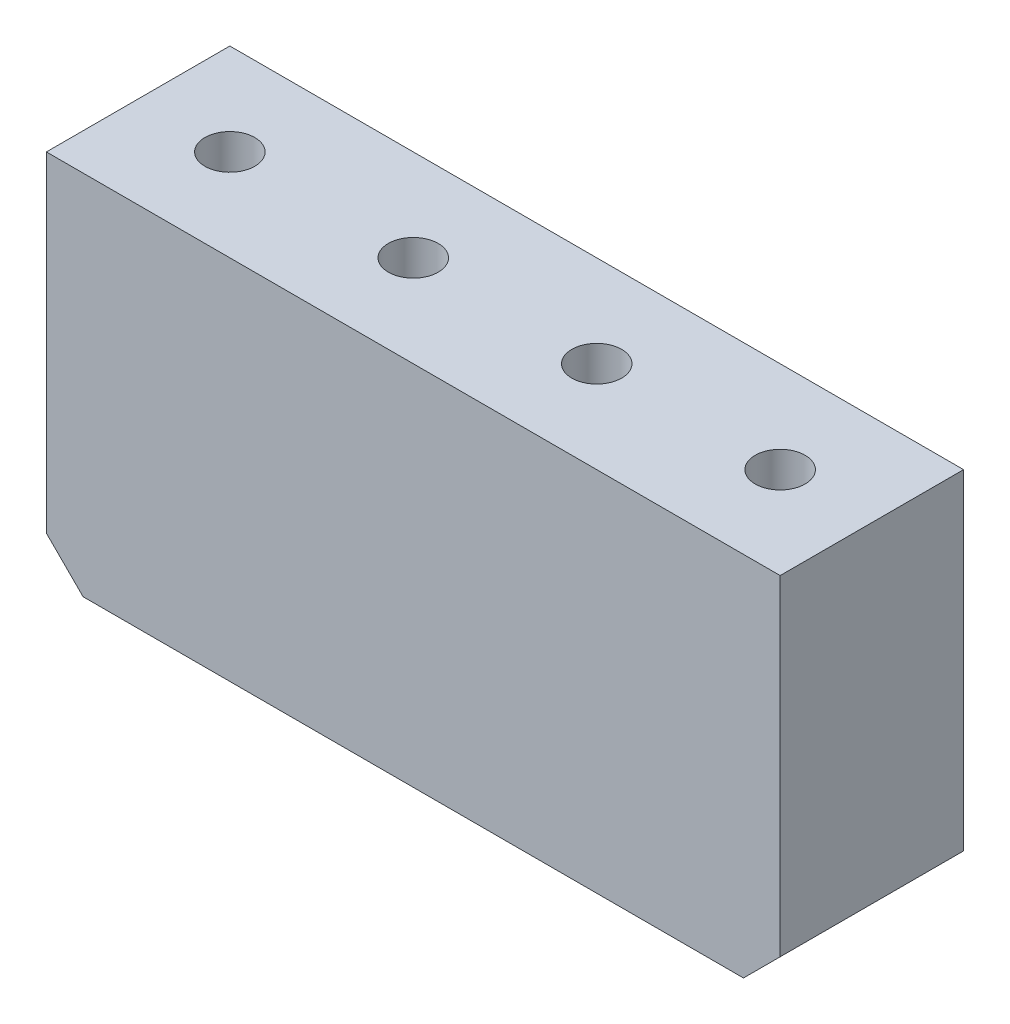
SolidWorks part; units mm, degrees
material "1023 碳钢板 (SS)"
ref_plane "Front Plane" through (0, 0, 0) normal (0, 0, 1) x (1, 0, 0)
ref_plane "Top Plane" through (0, 0, 0) normal (0, 1, 0) x (1, 0, 0)
ref_plane "Right Plane" through (0, 0, 0) normal (1, 0, 0) x (0, 0, -1)
sketch "Sketch1" plane through (0, 0, 0) normal (0, 0, 1) x (1, 0, 0)
  line L1 (-50, 25) -> (50, 25)
  line L2 (-50, 25) -> (-50, -25)
  line L3 (-50, -25) -> (50, -25)
  line L4 (50, 25) -> (50, -25)
  line L5 (-50, 25) -> (50, -25) construction
  line L6 (-50, -25) -> (50, 25) construction
  point P0 (0, 0)
  dimension "D1" = 100
  dimension "D2" = 50
extrude "Boss-Extrude1" add sketch "Sketch1" along normal blind 25 contours L2 L1 L4 L3
sketch "Sketch2" plane through (0, 25, 0) normal (0, 1, 0) x (1, 0, 0)
  line L0 (-50, -25) -> (-50, 0) construction
  circle A0 centre (-37.5, -12.5) radius 2.8145
  circle A1 centre (-12.5, -12.5) radius 3.8665
  circle A2 centre (37.5, -12.5) radius 5.7881
  circle A3 centre (12.5, -12.5) radius 3.4368
  point P12 (-50, -12.5)
  dimension "D1" = 25
  dimension "D2" = 25
  dimension "D3" = 75
  dimension "D4" = 12.5
hole_wizard "M8 Tapped Hole1" positions "Sketch3" profile "Sketch4" tap size "M8" standard "GB" end condition through all
sketch "Sketch3" plane through (0, 25, 0) normal (0, 1, 0) x (1, 0, 0)
  point P0 (-37.5, -12.5)
  point P3 (-12.5, -12.5)
  point P6 (12.5, -12.5)
  point P9 (37.5, -12.5)
cosmetic thread "Cosmetic thread 1" parameters "D2"=8
cosmetic thread "Cosmetic thread 2" parameters "D2"=8
cosmetic thread "Cosmetic thread 3" parameters "D2"=8
cosmetic thread "Cosmetic thread 4" parameters "D2"=8
sketch "Sketch4" plane through (-37.5, 25, 12.5) normal (1, 0, 0) x (0, 0, 1)
  line L0 (0, 0) -> (0, 50)
  line L1 (0, 50) -> (3.4, 50)
  line L2 (3.4, 50) -> (3.4, 0)
  line L5 (3.4, 0) -> (0, 0)
  line L11 (0, -6.35) -> (0, 107.95) construction
  dimension "通孔螺纹孔钻头直径" = 6.8
  dimension "通孔螺纹孔钻头深度" = 50
chamfer "Chamfer1" distance 5 angle 45 2 edges at (-50, -25, 12.5) (50, -25, 12.5)
